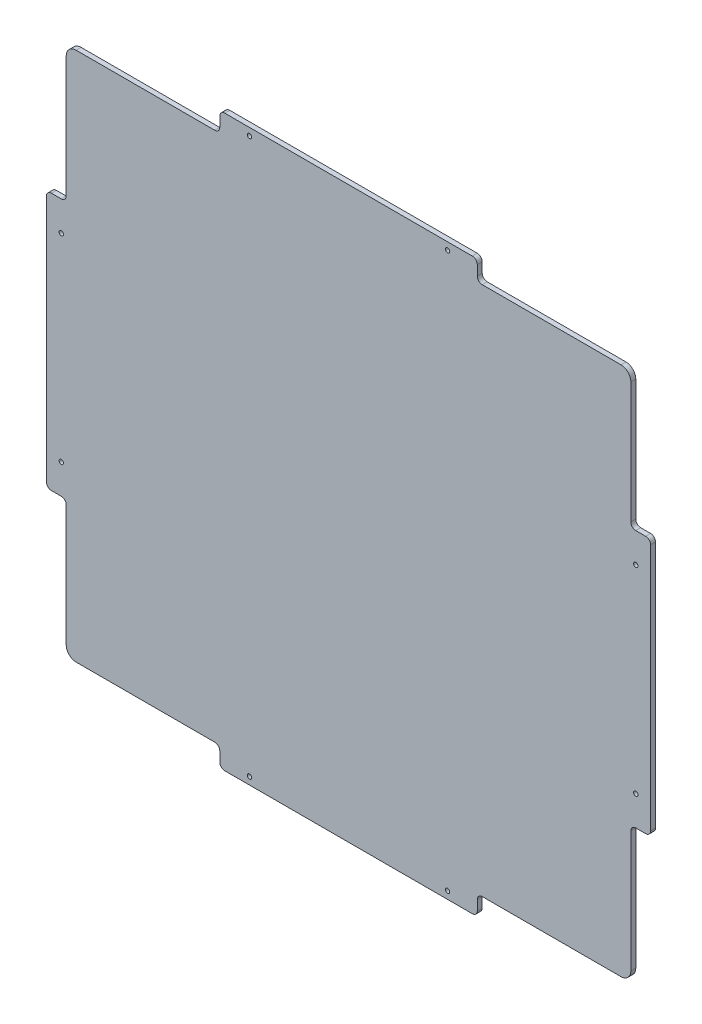
SolidWorks part; units mm, degrees
ref_plane "前视基准面" through (0, 0, 0) normal (0, 0, 1) x (1, 0, 0)
ref_plane "上视基准面" through (0, 0, 0) normal (0, 1, 0) x (1, 0, 0)
ref_plane "右视基准面" through (0, 0, 0) normal (1, 0, 0) x (0, 0, -1)
other "Configuration Table"
sketch "草图1" plane through (0, 0, 0) normal (0, 0, 1) x (1, 0, 0)
  line L1 (-285, 267.5) -> (285, 267.5)
  line L2 (-285, 267.5) -> (-285, -267.5)
  line L3 (-285, -267.5) -> (285, -267.5)
  line L4 (285, 267.5) -> (285, -267.5)
  line L5 (-285, 267.5) -> (285, -267.5) construction
  line L6 (-285, -267.5) -> (285, 267.5) construction
  point P0 (0, 0)
  dimension "D1" = 570
  dimension "D2" = 535
extrude "凸台-拉伸1" add sketch "草图1" along normal blind 5
fillet "圆角1" radius 10 4 edges at (-285, -267.5, 2.5) (285, -267.5, 2.5) (-285, 267.5, 2.5) (285, 267.5, 2.5)
sketch "草图4" plane through (0, 0, 0) normal (0, 0, -1) x (-1, 0, 0)
  line L0 (0, 0) -> (295, 0) construction
  line L1 (0, 0) -> (0, 298.1334) construction
  line L2 (-275, 267.5) -> (275, 267.5) construction
  line L3 (-130, 287.5) -> (130, 287.5)
  line L4 (-130, 287.5) -> (-130, 267.5)
  line L5 (-130, 267.5) -> (130, 267.5)
  line L6 (130, 287.5) -> (130, 267.5)
  line L7 (-130, 287.5) -> (130, 267.5) construction
  line L8 (-130, 267.5) -> (130, 287.5) construction
  line L9 (285, 257.5) -> (285, -257.5) construction
  line L10 (305, -130) -> (285, -130)
  line L11 (305, -130) -> (305, 130)
  line L12 (305, 130) -> (285, 130)
  line L13 (285, -130) -> (285, 130)
  line L14 (305, -130) -> (285, 130) construction
  line L15 (305, 130) -> (285, -130) construction
  line L16 (-130, -267.5) -> (130, -287.5) construction
  line L17 (-130, -287.5) -> (130, -267.5) construction
  line L18 (130, -287.5) -> (130, -267.5)
  line L19 (-130, -267.5) -> (130, -267.5)
  line L20 (-130, -287.5) -> (-130, -267.5)
  line L21 (-130, -287.5) -> (130, -287.5)
  line L22 (-305, 130) -> (-285, -130) construction
  line L23 (-305, -130) -> (-285, 130) construction
  line L24 (-285, -130) -> (-285, 130)
  line L25 (-305, 130) -> (-285, 130)
  line L26 (-305, -130) -> (-305, 130)
  line L27 (-305, -130) -> (-285, -130)
  point P2 (0, 277.5)
  point P17 (-121.8552, 287.5)
  point P22 (0, -277.5)
  dimension "D1" = 260
  dimension "D2" = 260
  dimension "D3" = 20
  dimension "D4" = 20
extrude "凸台-拉伸2" add sketch "草图4" against normal up to surface (5 mm away) up to face at (0, 0, 5)
sketch "草图5" plane through (0, 0, 0) normal (0, 0, -1) x (-1, 0, 0)
  line L0 (0, 0) -> (0, 303.2087) construction
  line L1 (0, 0) -> (340.026, 0) construction
  circle A0 centre (-100, 280) radius 2.2
  circle A1 centre (100, 280) radius 2.2
  circle A2 centre (290, 100) radius 2.2
  circle A3 centre (290, -100) radius 2.2
  circle A4 centre (100, -280) radius 2.2
  circle A5 centre (-100, -280) radius 2.2
  circle A6 centre (-290, -100) radius 2.2
  circle A7 centre (-290, 100) radius 2.2
  dimension "D1" = 4.4
  dimension "D2" = 200
  dimension "D3" = 200
  dimension "D4" = 560
  dimension "D5" = 580
extrude "切除-拉伸2" cut sketch "草图5" against normal through all
fillet "圆角2" radius 5 16 edges at (-130, 267.5, 2.5) (-130, 287.5, 2.5) (130, 267.5, 2.5) (285, 130, 2.5) (305, 130, 2.5) (305, -130, 2.5) (285, -130, 2.5) (130, -267.5, 2.5) (130, -287.5, 2.5) (-130, -287.5, 2.5) (-130, -267.5, 2.5) (-285, -130, 2.5) (-305, -130, 2.5) (-305, 130, 2.5) (-285, 130, 2.5) (130, 287.5, 2.5)
